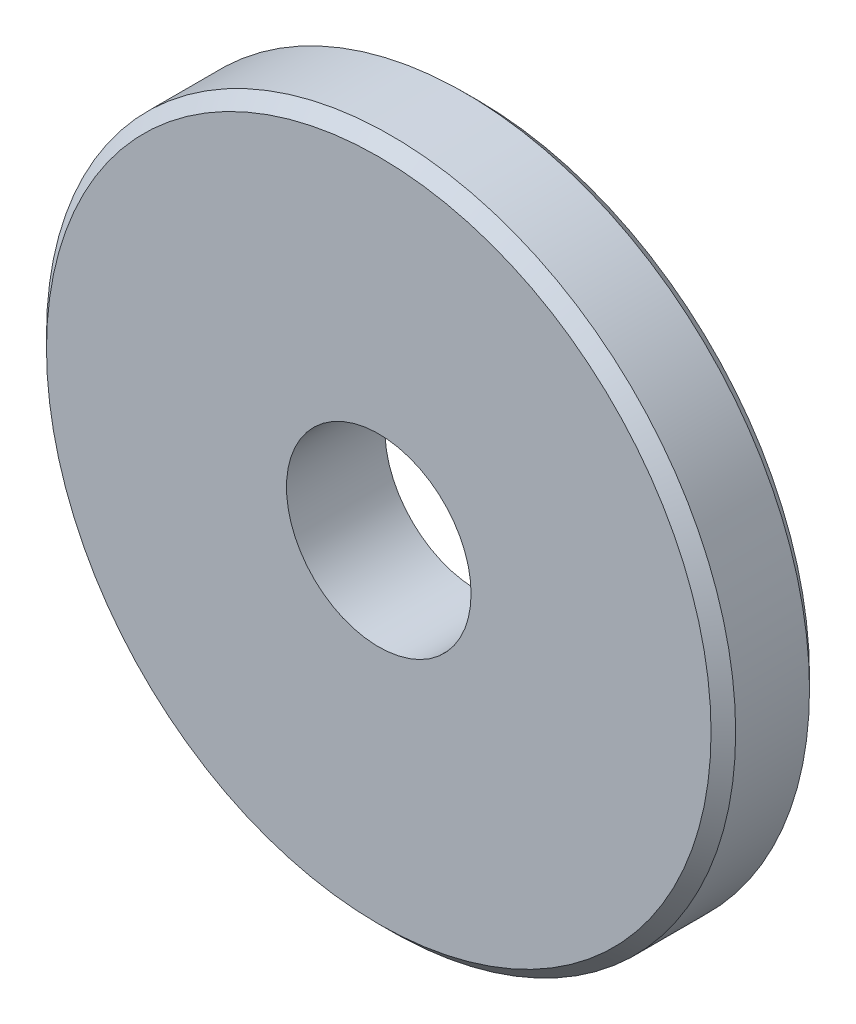
from build123d import *

# Parameters (mm, degrees)
SKETCH_1_R      = 28
SKETCH_1_R_2    = 7.5
EXTRUDE_1_DEPTH = 8
CHAMFER_1_SIZE  = 1


with BuildPart() as part:
    # 草图1 → 凸台-拉伸1 (new body)
    with BuildSketch(Plane.XY):
        Circle(SKETCH_1_R)
        Circle(SKETCH_1_R_2, mode=Mode.SUBTRACT)
    extrude(amount=EXTRUDE_1_DEPTH)

    # 倒角1
    chamfer_1_edges = [part.edges().sort_by_distance(p)[0] for p in [
        (-28, 0, 0),
        (-28, 0, 8),
    ]]
    chamfer(chamfer_1_edges, length=CHAMFER_1_SIZE)


solid = part.part
